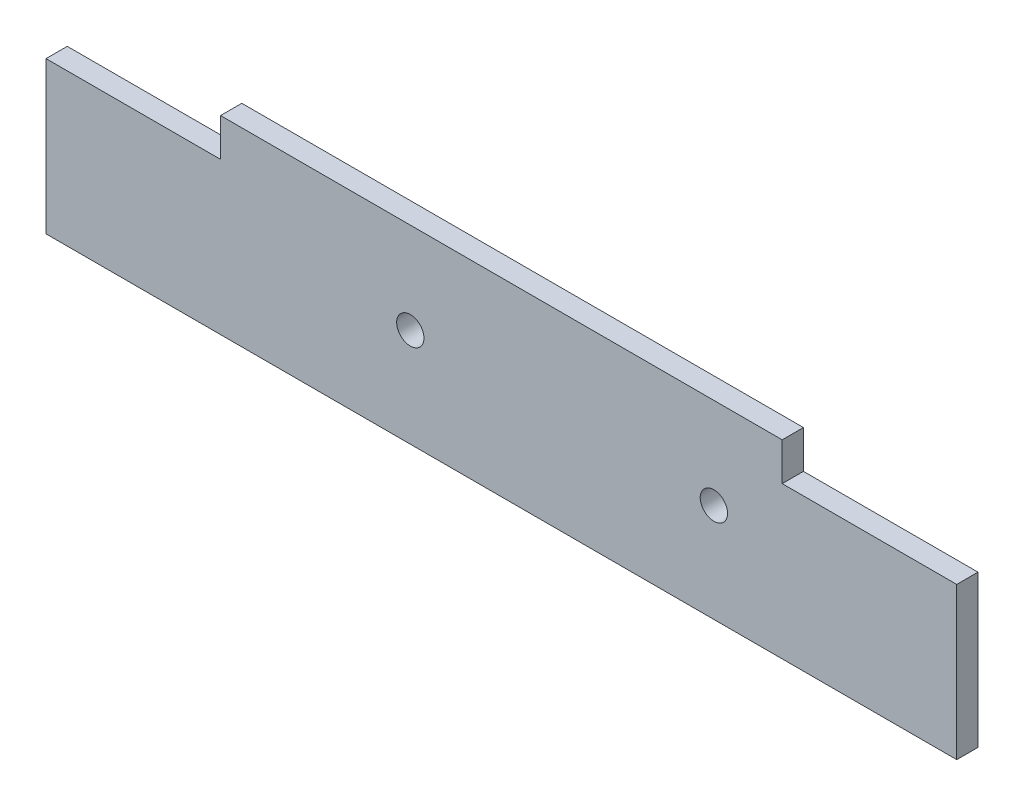
from build123d import *

# Parameters (mm, degrees)
SKETCH_1_R      = 9
EXTRUDE_1_DEPTH = 14


with BuildPart() as part:
    # 草图1 → 凸台-拉伸1 (new body)
    with BuildSketch(Plane.XY):
        Polygon((0, 0), (0, 100), (115, 100), (115, 125), (485, 125), (485, 100), (600, 100), (600, 0), align=None)
        with Locations((240, 65)):
            Circle(SKETCH_1_R, mode=Mode.SUBTRACT)
        with Locations((440, 65)):
            Circle(SKETCH_1_R, mode=Mode.SUBTRACT)
    extrude(amount=EXTRUDE_1_DEPTH)


solid = part.part
